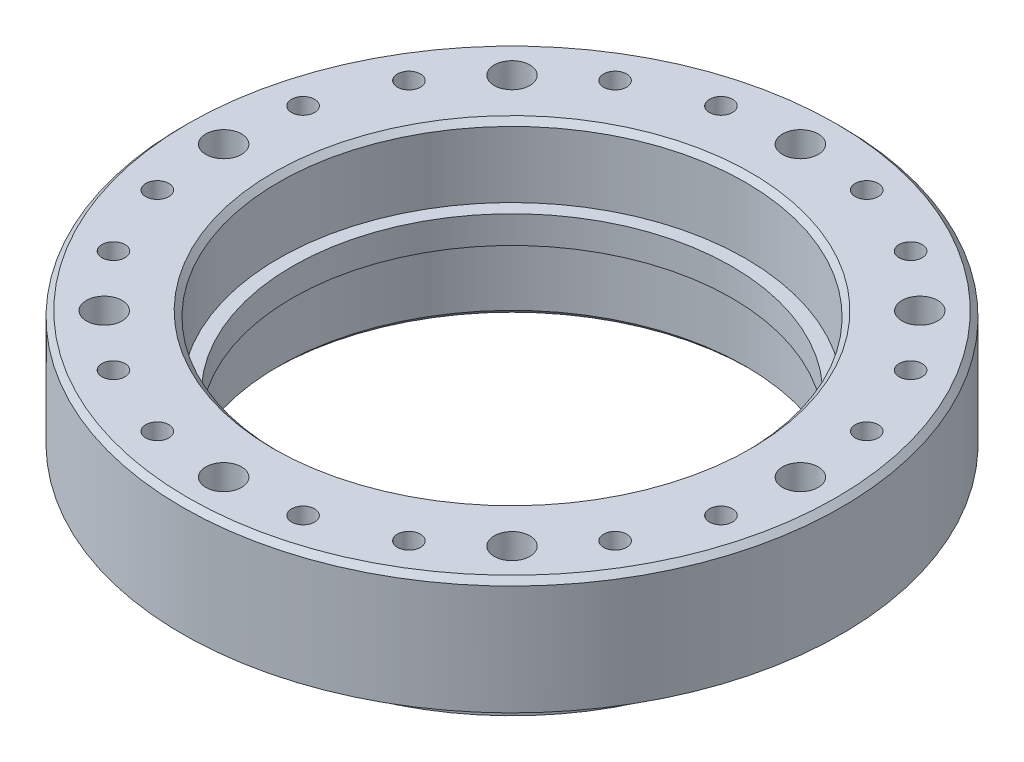
SolidWorks part; units mm, degrees
ref_plane "前视" through (0, 0, 0) normal (0, 0, 1) x (1, 0, 0)
ref_plane "上视" through (0, 0, 0) normal (0, 1, 0) x (1, 0, 0)
ref_plane "右视" through (0, 0, 0) normal (1, 0, 0) x (0, 0, -1)
sketch "草图1" plane through (0, 0, 0) normal (0, 1, 0) x (1, 0, 0)
  circle A0 centre (0, 0) radius 60
  circle A1 centre (0, 0) radius 40
  dimension "D1" = 120
  dimension "D2" = 80
extrude "凸台-拉伸1" add sketch "草图1" along normal mid plane 31
chamfer "倒角1" distance 1 angle 45 4 edges at (0, -15.5, 40) (0, -15.5, 60) (0, 15.5, 40) (0, 15.5, 60)
hole_wizard "打孔尺寸根据内六角圆柱头螺钉的类型1" positions "草图3" profile "草图2" counterbore size "M6" standard "Gb" end condition through all
sketch "草图3" plane through (-41.1264, -15.5, 15.0061) normal (0, 1, 0) x (1, 0, 0)
  line L0 (41.1264, 15.0061) -> (41.1264, 25.4816) construction
  line L2 (41.1264, 15.0061) -> (26.7637, 15.0061) construction
  point P0 (-11.3736, 15.0061)
  point P2 (93.6264, 15.0061)
  point P4 (41.1264, 67.5061)
  point P6 (41.1264, -37.4939)
  dimension "D1" = 105
  dimension "D2" = 105
sketch "草图2" plane through (-52.5, -15.5, 0) normal (1, 0, 0) x (0, 0, -1)
  line L0 (0, 0) -> (0, 31)
  line L1 (0, 31) -> (3.25, 31)
  line L3 (3.25, 31) -> (3.25, 6.8)
  line L4 (3.25, 6.8) -> (5.5, 6.8)
  line L5 (5.5, 6.8) -> (5.5, 0)
  line L7 (5.5, 0) -> (0, 0)
  line L11 (0, -6.35) -> (0, 107.95) construction
  dimension "通孔孔直径" = 6.5
  dimension "通孔孔深度" = 31
  dimension "柱形沉头孔直径" = 11
  dimension "柱形沉头孔深度" = 6.8
sketch "草图7" plane through (0, 15.5, 0) normal (0, 1, 0) x (1, 0, 0)
  circle A0 centre (0, 0) radius 42.5
  dimension "D1" = 85
extrude "切除-拉伸2" cut sketch "草图7" against normal blind 13
sketch "草图8" plane through (0, -15.5, 0) normal (0, -1, 0) x (1, 0, 0)
  circle A0 centre (0, 0) radius 42.5
  dimension "D1" = 85
extrude "切除-拉伸3" cut sketch "草图8" against normal blind 13
sketch "草图9" plane through (0, -15.5, 0) normal (0, -1, 0) x (1, 0, 0)
  circle A0 centre (0, 0) radius 46.5
  circle A1 centre (0, 0) radius 67.9942
  dimension "D1" = 93
extrude "切除-拉伸4" cut sketch "草图9" against normal blind 10
hole_wizard "M5 螺纹孔1" positions "草图6" profile "草图5" tap size "M5" standard "Gb" end condition through all
sketch "草图6" plane through (22.072, -5.5, -2.459) normal (0, -1, 0) x (-1, 0, 0)
  line L0 (-30.428, -2.459) -> (49969.572, -2.459) construction
  line L1 (22.072, -2.459) -> (22.072, -50002.459) construction
  line L2 (22.072, -2.459) -> (-46171.9046, 19131.7126) construction
  circle A0 centre (22.072, -2.459) radius 53 construction
  point P6 (-23.5943, 24.4405)
  point P9 (-29.2398, 10.8112)
  dimension "D1" = 106
  dimension "D2" = 22.5
  dimension "D3" = 14.7523
sketch "草图5" plane through (45.6663, -5.5, -26.8995) normal (1, 0, 0) x (0, 0, -1)
  line L0 (0, 0) -> (0, 21)
  line L1 (0, 21) -> (2.1, 21)
  line L2 (2.1, 21) -> (2.1, 0)
  line L5 (2.1, 0) -> (0, 0)
  line L11 (0, -6.35) -> (0, 107.95) construction
  dimension "通孔螺纹孔钻头直径" = 4.2
  dimension "通孔螺纹孔钻头深度" = 21
cosmetic thread "孔螺蚊线1" parameters "D2"=5
cosmetic thread "孔螺蚊线2" parameters "D2"=5
pattern_circular "阵列(圆周)1" count 8 every 45 about axis through (0, 0, 0) along (0, 1, 0) of "M5 螺纹孔1"
sketch "草图10" plane through (0, -5.5, 0) normal (0, -1, 0) x (1, 0, 0)
  circle A0 centre (0, -52.5) radius 6
  circle A1 centre (52.5, 0) radius 6
  circle A2 centre (0, 52.5) radius 6
  circle A3 centre (-52.5, 0) radius 6
  dimension "D1" = 12
extrude "切除-拉伸5" cut sketch "草图10" against normal blind 10
pattern_circular "阵列(圆周)2" count 2 every 45 about axis through (0, 0, 0) along (0, 1, 0) of "打孔尺寸根据内六角圆柱头螺钉的类型1"
pattern_circular "阵列(圆周)3" count 2 every 45 about axis through (0, 0, 0) along (0, 1, 0) of "切除-拉伸5"
chamfer "倒角2" distance 1 angle 45 2 edges at (0, 15.5, 42.5) (0, -15.5, -42.5)
